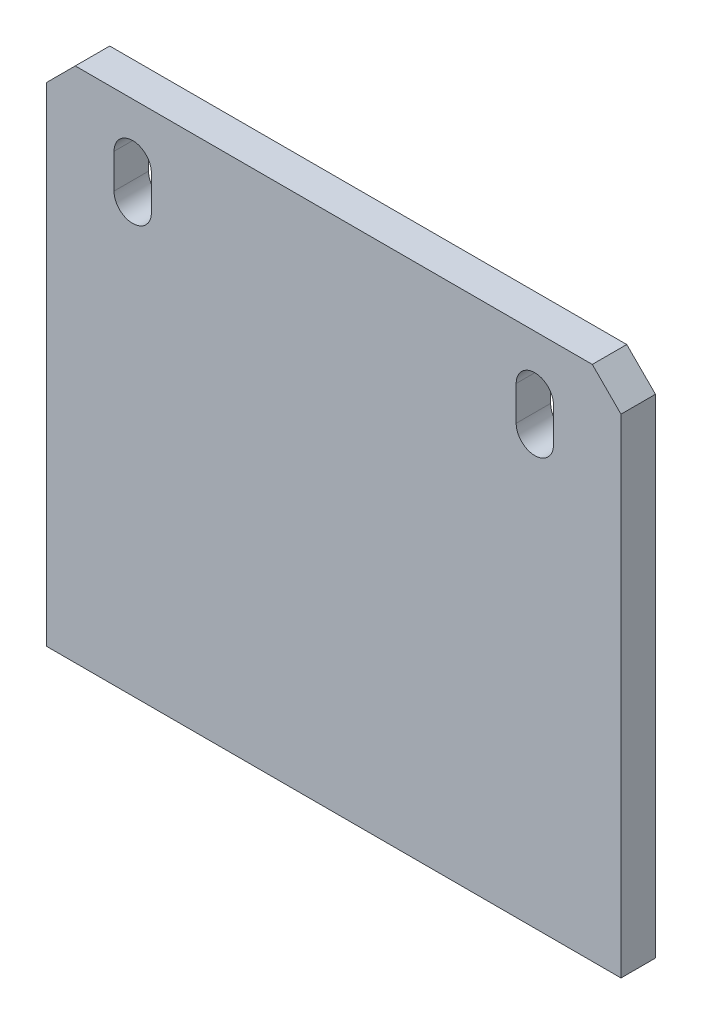
SolidWorks part; units mm, degrees
material "1023 碳钢板 (SS)"
ref_plane "Front Plane" through (0, 0, 0) normal (0, 0, 1) x (1, 0, 0)
ref_plane "Top Plane" through (0, 0, 0) normal (0, 1, 0) x (1, 0, 0)
ref_plane "Right Plane" through (0, 0, 0) normal (1, 0, 0) x (0, 0, -1)
sketch "Sketch1" plane through (0, 0, 0) normal (0, 0, 1) x (1, 0, 0)
  line L1 (100, 90) -> (-100, 90)
  line L2 (100, 90) -> (100, -90)
  line L3 (100, -90) -> (-100, -90)
  line L4 (-100, 90) -> (-100, -90)
  line L5 (100, 90) -> (-100, -90) construction
  line L6 (100, -90) -> (-100, 90) construction
  point P0 (0, 0)
  dimension "D1" = 200
  dimension "D2" = 180
extrude "Boss-Extrude1" add sketch "Sketch1" along normal blind 12 contours L2 L1 L4 L3
chamfer "Chamfer1" distance 10 angle 45 2 edges at (-100, 90, 6) (100, 90, 6)
sketch "Sketch2" plane through (0, 0, 12) normal (0, 0, 1) x (1, 0, 0)
  line L0 (-70, 71) -> (-70, 59) construction
  line L1 (-63.5, 71) -> (-63.5, 59)
  line L2 (-76.5, 71) -> (-76.5, 59)
  line L3 (70, 71) -> (70, 59) construction
  line L4 (76.5, 71) -> (76.5, 59)
  line L5 (63.5, 71) -> (63.5, 59)
  line L6 (90, 90) -> (-90, 90) construction
  arc A0 (-63.5, 71) -> (-76.5, 71) centre (-70, 71) ccw
  arc A1 (-76.5, 59) -> (-63.5, 59) centre (-70, 59) ccw
  arc A2 (76.5, 71) -> (63.5, 71) centre (70, 71) ccw
  arc A3 (63.5, 59) -> (76.5, 59) centre (70, 59) ccw
  point P2 (-70, 65)
  point P7 (70, 65)
  dimension "D1" = 6.5
  dimension "D3" = 140
  dimension "D2" = 12
  dimension "D4" = 70
  dimension "D5" = 25
extrude "Cut-Extrude1" cut sketch "Sketch2" against normal blind 12
